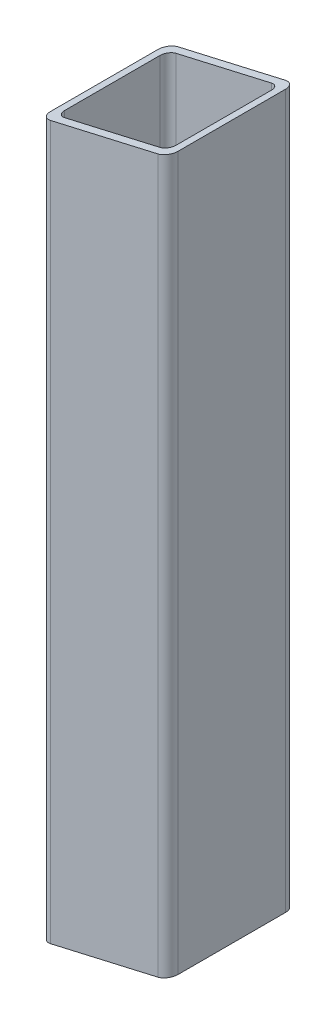
from build123d import *

# Parameters (mm, degrees)
BOSS_EXTRUDE1_DEPTH = 291
CUT_EXTRUDE1_REACH  = 325.544


with BuildPart() as part:
    # Sketch2 → Boss-Extrude1 (new, symmetric)
    with BuildSketch(Plane(origin=(0, 0, 0), x_dir=(1, 0, 0), z_dir=(0, 1, 0))):
        with BuildLine():
            Line((7.875, -1.525), (92.125, -1.525))
            ThreePointArc((92.125, -1.525), (97.693465902, 0.781534098), (100, 6.35))
            Line((100, 6.35), (100, 90.6))
            ThreePointArc((100, 90.6), (97.693465902, 96.168465902), (92.125, 98.475))
            Line((92.125, 98.475), (7.875, 98.475))
            ThreePointArc((7.875, 98.475), (2.306534098, 96.168465902), (0, 90.6))
            Line((0, 90.6), (0, 6.35))
            ThreePointArc((0, 6.35), (2.306534098, 0.781534098), (7.875, -1.525))
        make_face()
        with BuildLine():
            Line((12.6, 4.775), (87.4, 4.775))
            ThreePointArc((87.4, 4.775), (91.854772721, 6.620227279), (93.7, 11.075))
            Line((93.7, 11.075), (93.7, 85.875))
            ThreePointArc((93.7, 85.875), (91.854772721, 90.329772721), (87.4, 92.175))
            Line((87.4, 92.175), (12.6, 92.175))
            ThreePointArc((12.6, 92.175), (8.145227279, 90.329772721), (6.3, 85.875))
            Line((6.3, 85.875), (6.3, 11.075))
            ThreePointArc((6.3, 11.075), (8.145227279, 6.620227279), (12.6, 4.775))
        make_face(mode=Mode.SUBTRACT)
    extrude(amount=BOSS_EXTRUDE1_DEPTH, both=True)

    # Sketch4 → Cut-Extrude1 (cut, up to next)
    with BuildSketch(Plane.XY.offset(1.525), mode=Mode.PRIVATE) as cut_extrude1_sk1:
        Polygon((100, 291), (0, 268), (0, 291), align=None)
    cut_extrude1_tool1 = extrude(cut_extrude1_sk1.sketch, amount=-CUT_EXTRUDE1_REACH, mode=Mode.PRIVATE) & part.part
    # Sketch4 → Cut-Extrude1 (cut, up to next)
    with BuildSketch(Plane.XY.offset(1.525), mode=Mode.PRIVATE) as cut_extrude1_sk2:
        Polygon((0, -291), (100, -268), (100, -291), align=None)
    cut_extrude1_tool2 = extrude(cut_extrude1_sk2.sketch, amount=-CUT_EXTRUDE1_REACH, mode=Mode.PRIVATE) & part.part
    add(cut_extrude1_tool1.solids().sort_by_distance((33.333333, 283.333333, 1.525))[0], mode=Mode.SUBTRACT)
    add(cut_extrude1_tool2.solids().sort_by_distance((66.666667, -283.333333, 1.525))[0], mode=Mode.SUBTRACT)


solid = part.part
